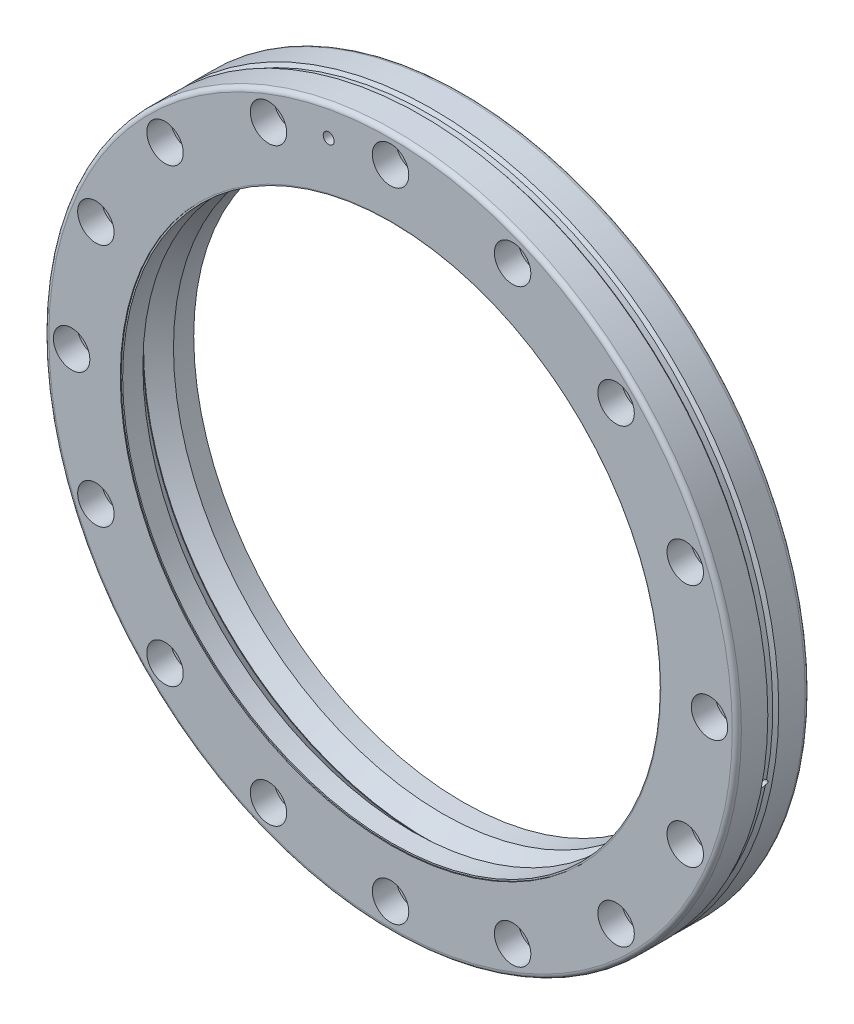
from build123d import *

# Parameters (mm, degrees)
SKETCH_1_R                     = 190
SKETCH_1_R_2                   = 147.5
EXTRUDE_1_DEPTH                = 20
FILLET_1_R                     = 2.5
HOLE_WIZARD_M1_6_1_D           = 14
HOLE_WIZARD_M1_6_1_CBORE_D     = 20
HOLE_WIZARD_M1_6_1_CBORE_DEPTH = 13
PATTERN_CIRCULAR_1_COUNT       = 16
CUT_EXTRUDE_START              = 190
SKETCH_7_R                     = 2
CUT_EXTRUDE_1_DEPTH            = 5
SKETCH_8_R                     = 0.5
CUT_EXTRUDE_2_DEPTH            = 15
PATTERN_CIRCULAR_2_COUNT       = 2
SKETCH_9_R                     = 148.3
CUT_EXTRUDE_3_DEPTH            = 0.5


with BuildPart() as part:
    # 草图1 → 凸台-拉伸1 (new, symmetric)
    with BuildSketch(Plane.XY):
        Circle(SKETCH_1_R)
        Circle(SKETCH_1_R_2, mode=Mode.SUBTRACT)
    extrude(amount=EXTRUDE_1_DEPTH, both=True)

    # 草图2 → 切除-旋转1 (revolve, cut)
    with BuildSketch(Plane(origin=(0, 0, 0), x_dir=(0, 0, -1), z_dir=(1, 0, 0)), mode=Mode.PRIVATE) as cut_revolve_1_sk:
        with BuildLine():
            Line((-8.485281374, 147.4), (-0.176776695, 155.708504679))
            ThreePointArc((-0.176776695, 155.708504679), (0, 156.135281374), (0.176776695, 155.708504679))
            Line((0.176776695, 155.708504679), (8.485281374, 147.4))
            Line((8.485281374, 147.4), (-8.485281374, 147.4))
        make_face()
        Polygon((-3, 190), (3, 190), (1.5, 188.2), (-1.5, 188.2), align=None)
    revolve(cut_revolve_1_sk.sketch.rotate(Axis((0, 0, 12.553599724), (0, 0, -1)), 90), axis=Axis((0, 0, 12.553599724), (0, 0, -1)), mode=Mode.SUBTRACT)

    # 圆角1
    fillet_1_edges = [part.edges().sort_by_distance(p)[0] for p in [
        (-190, 0, -20),
        (-190, 0, 20),
    ]]
    fillet(fillet_1_edges, radius=FILLET_1_R)

    # M1.6 六角头螺栓的柱形沉头孔1 (through all)
    with Locations(Plane.XY.offset(20)):
        with Locations((0, 175)):
            hole_wizard_m1_6_1 = CounterBoreHole(HOLE_WIZARD_M1_6_1_D / 2, HOLE_WIZARD_M1_6_1_CBORE_D / 2, HOLE_WIZARD_M1_6_1_CBORE_DEPTH)

    # 阵列(圆周)1: M1.6 六角头螺栓的柱形沉头孔1 ×16 about axis
    pattern_circular_1_axis = Axis((0, 0, 0), (0, 0, 1))
    for i in range(1, PATTERN_CIRCULAR_1_COUNT):
        add(hole_wizard_m1_6_1.rotate(pattern_circular_1_axis, i * 360 / PATTERN_CIRCULAR_1_COUNT), mode=Mode.SUBTRACT)

    # 草图7 → 切除-拉伸1 (cut)
    with BuildSketch(Plane(origin=(0, 0, 0), x_dir=(0, 0, -1), z_dir=(0.9807852804032297, -0.19509032201613213, 0)).offset(CUT_EXTRUDE_START)):
        with Locations(Location((0, 0, 0), (0, 0, 90))):
            Circle(SKETCH_7_R)
    cut_extrude_1 = extrude(amount=-CUT_EXTRUDE_1_DEPTH, mode=Mode.SUBTRACT)

    # 草图8 → 切除-拉伸2 (cut)
    with BuildSketch(Plane(origin=(181.445276875, -36.091709573, 0), x_dir=(-0.19509032201613213, -0.9807852804032298, 0), z_dir=(0.9807852804032297, -0.1950903220161321, 0))):
        with Locations(Location((0, 0, 0), (0, 0, 180))):
            Circle(SKETCH_8_R)
    cut_extrude_2 = extrude(amount=-CUT_EXTRUDE_2_DEPTH, mode=Mode.SUBTRACT)

    # 阵列(圆周)2: 切除-拉伸1, 切除-拉伸2 ×2 about axis
    pattern_circular_2_axis = Axis((0, 0, 20), (0, 0, -1))
    add([cut_extrude_1.rotate(pattern_circular_2_axis, i * 360 / PATTERN_CIRCULAR_2_COUNT) for i in range(1, PATTERN_CIRCULAR_2_COUNT)], mode=Mode.SUBTRACT)
    add([cut_extrude_2.rotate(pattern_circular_2_axis, i * 360 / PATTERN_CIRCULAR_2_COUNT) for i in range(1, PATTERN_CIRCULAR_2_COUNT)], mode=Mode.SUBTRACT)

    # 草图9 → 切除-拉伸3 (cut)
    with BuildSketch(Plane.XY.offset(20)):
        Circle(SKETCH_9_R)
    cut_extrude_3 = extrude(amount=-CUT_EXTRUDE_3_DEPTH, mode=Mode.SUBTRACT)

    # 镜向1: 切除-拉伸3 across plane
    add(cut_extrude_3.mirror(Plane.XY), mode=Mode.SUBTRACT)

    # 切除-拉伸4 cone 1 section (through the dimple's axis) → 切除-拉伸4 (revolve, cut)
    with BuildSketch(Plane(origin=(-33.945716031, 170.65663879, 20), x_dir=(0, -1, 0), z_dir=(1, 0, 0))):
        Polygon((0, 0), (3, 0), (0, 150.758469861), align=None)
    revolve(axis=Axis((-33.945716031, 170.65663879, 20), (0, 0, -1)), mode=Mode.SUBTRACT)


solid = part.part
